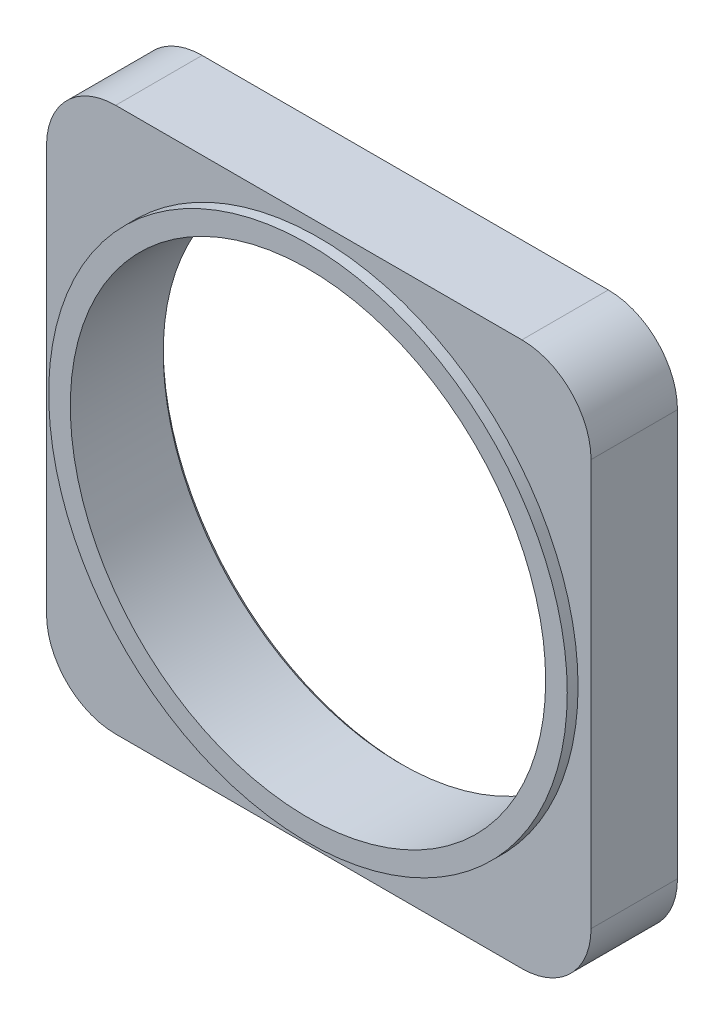
from build123d import *

# Parameters (mm, degrees)
SKETCH1_R                  = 55
BOSS_EXTRUDE1_DEPTH        = 20
SKETCH2_R                  = 60
SKETCH2_R_2                = 55
BOSS_EXTRUDE2_DEPTH        = 2.5
M10X1_5_TAPPED_HOLE1_D     = 8.5
M10X1_5_TAPPED_HOLE1_DEPTH = 12
M10X1_5_TAPPED_HOLE1_TIP   = 2.553657631
CHAMFER1_SIZE              = 1


with BuildPart() as part:
    # Sketch1 → Boss-Extrude1 (new body)
    with BuildSketch(Plane.XY):
        with BuildLine():
            Line((16, 0), (110, 0))
            ThreePointArc((110, 0), (121.313708499, 4.686291501), (126, 16))
            Line((126, 16), (126, 110))
            ThreePointArc((126, 110), (121.313708499, 121.313708499), (110, 126))
            Line((110, 126), (16, 126))
            ThreePointArc((16, 126), (4.686291501, 121.313708499), (0, 110))
            Line((0, 110), (0, 16))
            ThreePointArc((0, 16), (4.686291501, 4.686291501), (16, 0))
        make_face()
        with Locations((63, 63)):
            Circle(SKETCH1_R, mode=Mode.SUBTRACT)
    extrude(amount=BOSS_EXTRUDE1_DEPTH)

    # Sketch2 → Boss-Extrude2 (add)
    with BuildSketch(Plane.XY.offset(20)):
        with Locations((63, 63)):
            Circle(SKETCH2_R)
        with Locations((63, 63)):
            Circle(SKETCH2_R_2, mode=Mode.SUBTRACT)
    extrude(amount=BOSS_EXTRUDE2_DEPTH)

    # M10x1.5 Tapped Hole1
    with Locations(Plane(origin=(110, 110, 0), x_dir=(-1, 0, 0), z_dir=(0, 0, -1))):
        with Locations((0, 0), (94, 0), (94, -94), (0, -94)):
            Hole(M10X1_5_TAPPED_HOLE1_D / 2, depth=M10X1_5_TAPPED_HOLE1_DEPTH)
            with Locations((0, 0, -(M10X1_5_TAPPED_HOLE1_DEPTH + M10X1_5_TAPPED_HOLE1_TIP / 2))):  # 118° drill point
                Cone(0, M10X1_5_TAPPED_HOLE1_D / 2, M10X1_5_TAPPED_HOLE1_TIP, mode=Mode.SUBTRACT)

    # Chamfer1
    chamfer1_edges = [part.edges().sort_by_distance(p)[0] for p in [
        (8, 63, 0),
    ]]
    chamfer(chamfer1_edges, length=CHAMFER1_SIZE)


solid = part.part
